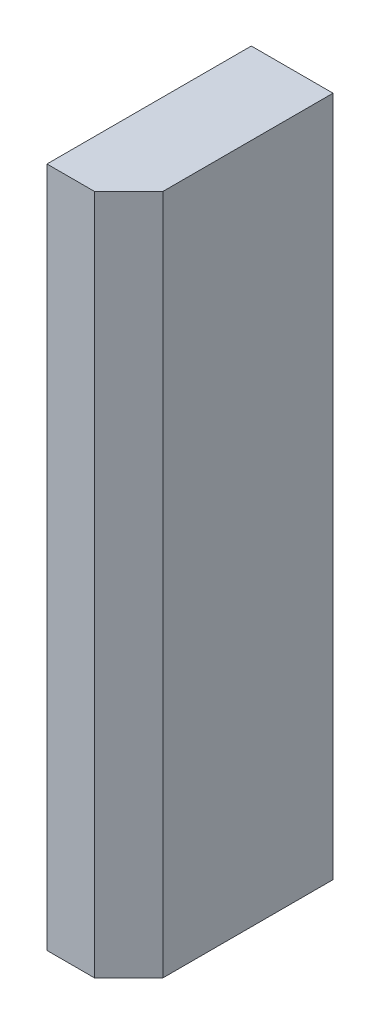
SolidWorks part; units mm, degrees
ref_plane "Front Plane" through (0, 0, 0) normal (0, 0, 1) x (1, 0, 0)
ref_plane "Top Plane" through (0, 0, 0) normal (0, 1, 0) x (1, 0, 0)
ref_plane "Right Plane" through (0, 0, 0) normal (1, 0, 0) x (0, 0, -1)
sketch "Sketch1" plane through (0, 0, 0) normal (0, 0, 1) x (1, 0, 0)
  line L1 (-60, 500) -> (60, 500)
  line L2 (-60, 500) -> (-60, -500)
  line L3 (-60, -500) -> (60, -500)
  line L4 (60, 500) -> (60, -500)
  line L5 (-60, 500) -> (60, -500) construction
  line L6 (-60, -500) -> (60, 500) construction
  point P0 (0, 0)
  dimension "D1" = 1000
  dimension "D2" = 120
extrude "Boss-Extrude1" add sketch "Sketch1" along normal blind 300
chamfer "Chamfer1" distance 50 angle 45 1 edges at (60, 0, 300)
